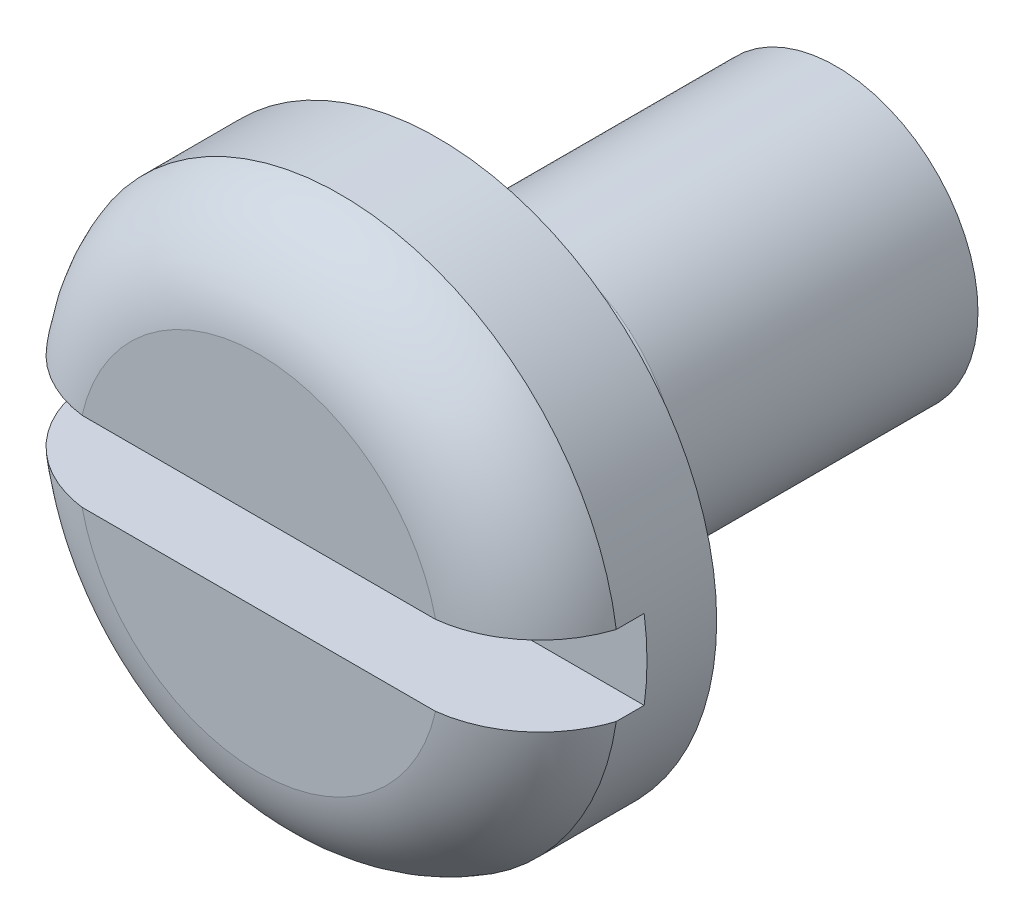
from build123d import *

# Parameters (mm, degrees)
SKETCH_1_R           = 2.8
BOSS_EXTRUDE_1_DEPTH = 1.8
SKETCH_4_R           = 1.375
BOSS_EXTRUDE_2_DEPTH = 0.7
SKETCH_6_R           = 1.425
BOSS_EXTRUDE_3_DEPTH = 3
SKETCH_8_W           = 1.368195424
SKETCH_8_H           = 0.8
CUT_EXTRUDE_1_DEPTH  = 8.429670248


with BuildPart() as part:
    # Sketch 1 → Boss-Extrude 1 (new body)
    with BuildSketch(Plane.XY):
        Circle(SKETCH_1_R)
    extrude(amount=BOSS_EXTRUDE_1_DEPTH)

    # Sketch 3 → Revolve 1 (revolve)
    with BuildSketch(Plane(origin=(0, 0, 0), x_dir=(1, 0, 0), z_dir=(0, 1, 0))):
        with BuildLine():
            Line((0, 0), (1.475, 0))
            ThreePointArc((1.475, 0), (1.42299689, 0.04799689), (1.375, 0.1))
            Line((1.375, 0.1), (0, 0.1))
            Line((0, 0.1), (0, 0))
        make_face()
    revolve(axis=Axis((0, 0, 0), (0, 0, -1)))

    # Sketch 4 → Boss-Extrude 2 (add)
    with BuildSketch(Plane(origin=(0, 0, -0.1), x_dir=(-1, 0, 0), z_dir=(0, 0, -1))):
        Circle(SKETCH_4_R)
    extrude(amount=BOSS_EXTRUDE_2_DEPTH)

    # Sketch 5 → Revolve 2 (revolve)
    with BuildSketch(Plane(origin=(0, 0, 0), x_dir=(1, 0, 0), z_dir=(0, 1, 0)), mode=Mode.PRIVATE) as revolve_2_sk:
        Polygon((0, 0.8), (1.375, 0.8), (1.425, 1), (0, 1), align=None)
    revolve(revolve_2_sk.sketch.rotate(Axis((0, 0, 0), (0, 0, -1)), 180), axis=Axis((0, 0, 0), (0, 0, -1)))

    # Sketch 6 → Boss-Extrude 3 (add)
    with BuildSketch(Plane(origin=(0, 0, -1), x_dir=(-1, 0, 0), z_dir=(0, 0, -1))):
        Circle(SKETCH_6_R)
    extrude(amount=BOSS_EXTRUDE_3_DEPTH)

    # Sketch 7 → Cut-Revolve 3 (revolve, cut)
    with BuildSketch(Plane(origin=(0, 0, 0), x_dir=(1, 0, 0), z_dir=(0, 1, 0)), mode=Mode.PRIVATE) as cut_revolve_3_sk:
        with BuildLine():
            Line((1.82, -1.8), (2.8, -1.8))
            Line((2.8, -1.8), (2.8, -0.98))
            ThreePointArc((2.8, -0.98), (2.429916567, -1.533314921), (1.82, -1.8))
        make_face()
    revolve(cut_revolve_3_sk.sketch.rotate(Axis((0, 0, -0.11680497), (0, 0, 1)), 180), axis=Axis((0, 0, -0.11680497), (0, 0, 1)), mode=Mode.SUBTRACT)

    # Sketch 8 → Cut-Extrude 1 (cut, through all)
    with BuildSketch(Plane.ZY.offset(2.8)):
        with Locations((1.384097712, 0)):
            Rectangle(SKETCH_8_W, SKETCH_8_H)
    extrude(amount=-CUT_EXTRUDE_1_DEPTH, mode=Mode.SUBTRACT)


solid = part.part
